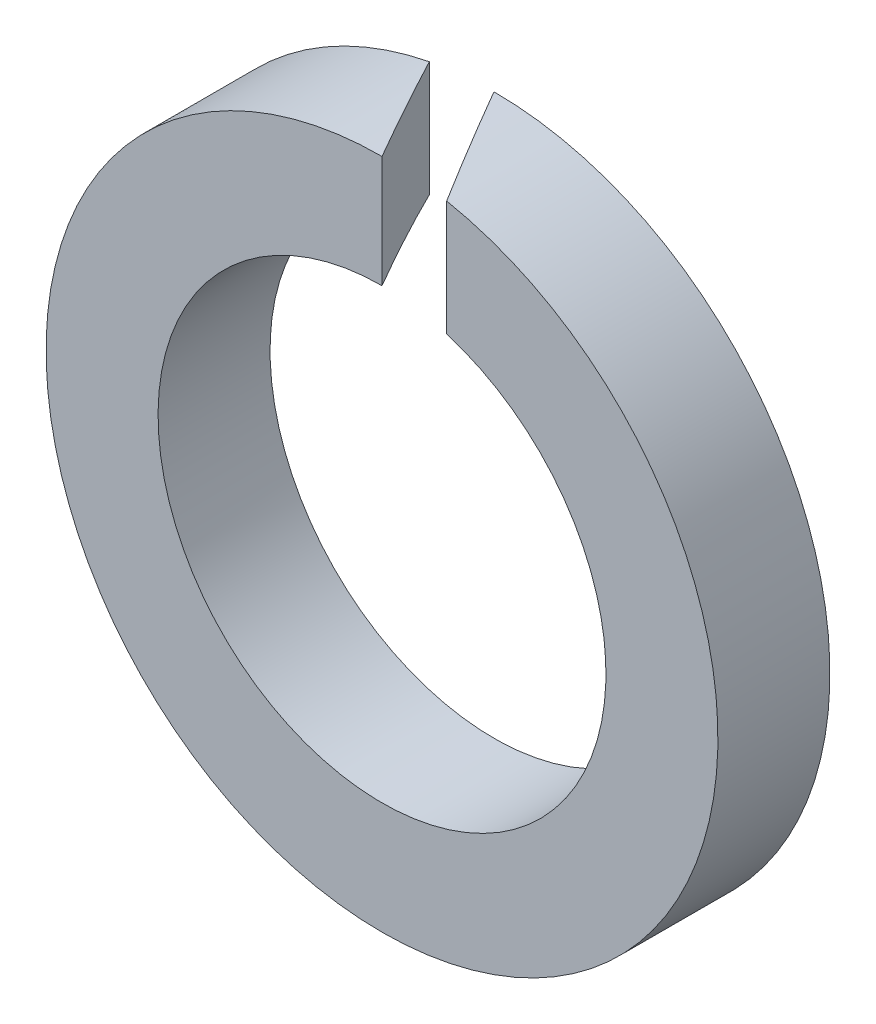
from build123d import *

# Parameters (mm, degrees)
SKETCH1_R          = 3.3
SKETCH1_R_2        = 2.2
BASE_EXTRUDE_DEPTH = 1.1
CUT_EXTRUDE1_DEPTH = 5.794788838


with BuildPart() as part:
    # Sketch1 → Base-Extrude (new body)
    with BuildSketch(Plane.XY):
        Circle(SKETCH1_R)
        Circle(SKETCH1_R_2, mode=Mode.SUBTRACT)
    extrude(amount=-BASE_EXTRUDE_DEPTH)

    # Sketch2 → Cut-Extrude1 (cut, through all)
    with BuildSketch(Plane(origin=(0, 0, 0), x_dir=(1, 0, 0), z_dir=(0, 1, 0))):
        Polygon((0, 1.1), (0.635085296, 0), (0, 0), (-0.635085296, 1.1), align=None)
    extrude(amount=CUT_EXTRUDE1_DEPTH, mode=Mode.SUBTRACT)


solid = part.part
